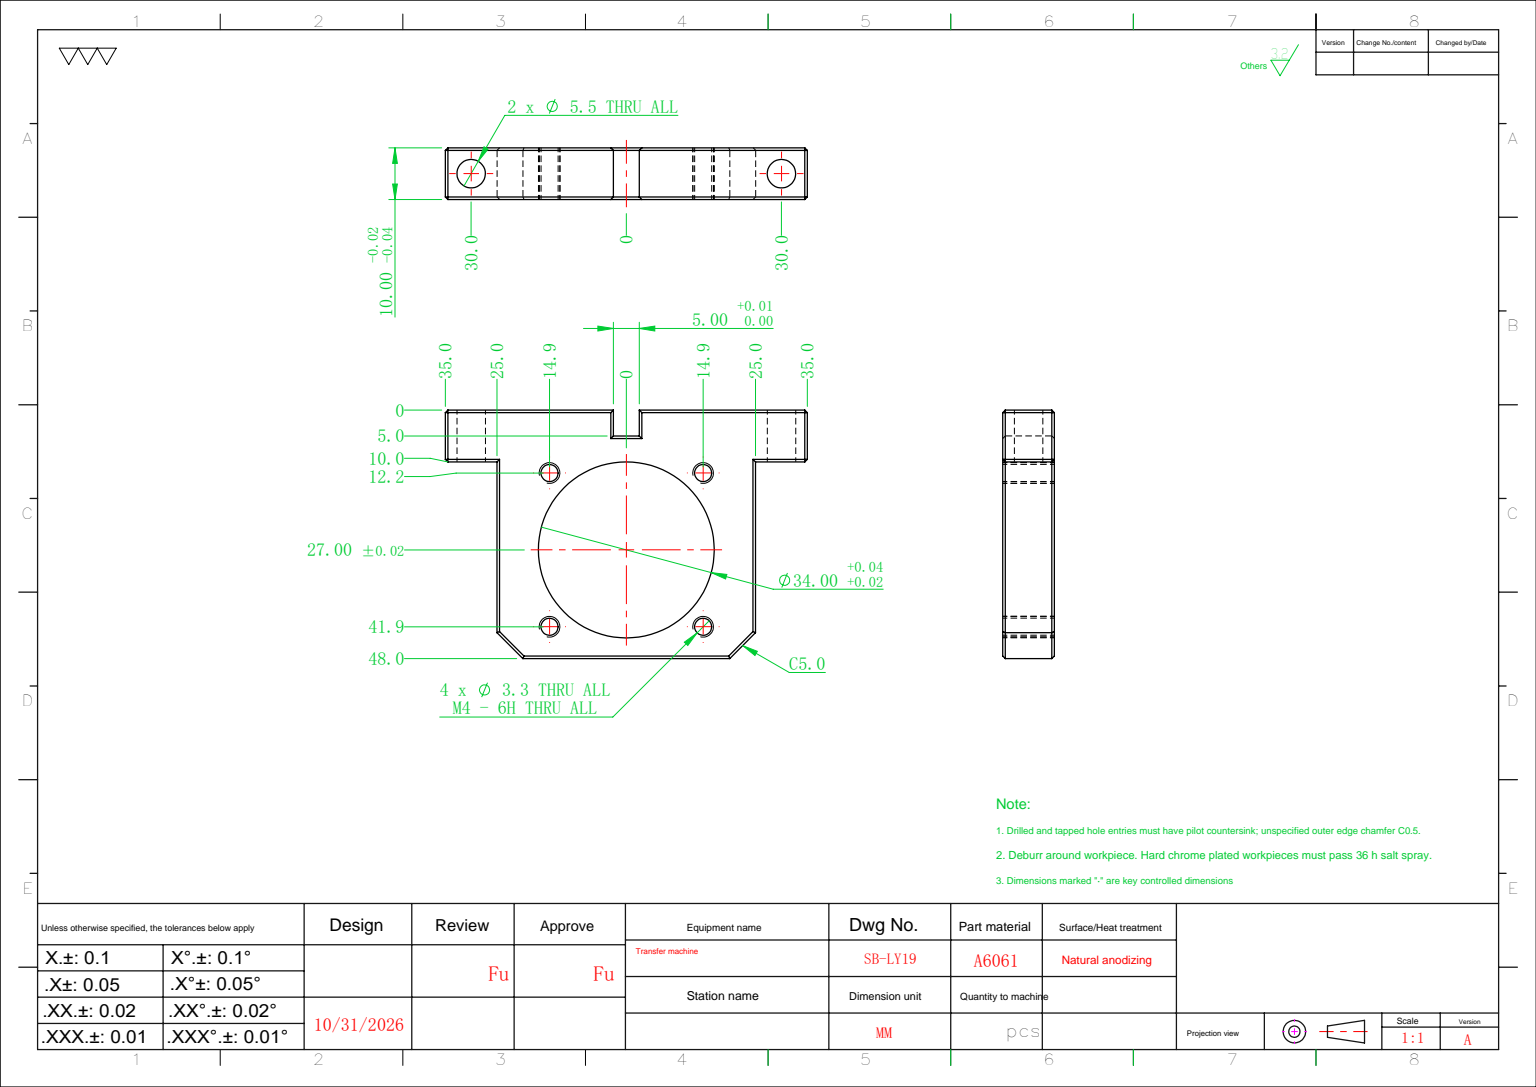
from build123d import *

# Parameters (mm, degrees)
SKETCH_1_W              = 70
SKETCH_1_H              = 48
EXTRUDE_1_DEPTH         = 10
SKETCH_2_W              = 10
SKETCH_2_H              = 38
CUT_EXTRUDE_1_DEPTH     = 44.600458713
SKETCH_3_R              = 17
CUT_EXTRUDE_2_DEPTH     = 44.600458713
HOLE_WIZARD_M4_2_D      = 3.3
HOLE_WIZARD_5_5_5_5_1_D = 5.5
CHAMFER_1_SIZE          = 5
SKETCH_12_W             = 5
SKETCH_12_H             = 5
CUT_EXTRUDE_3_DEPTH     = 44.600458713
CHAMFER_2_SIZE          = 0.5


with BuildPart() as part:
    # 草图1 → 凸台-拉伸1 (new body)
    with BuildSketch(Plane.XY):
        Rectangle(SKETCH_1_W, SKETCH_1_H)
    extrude(amount=EXTRUDE_1_DEPTH)

    # 草图2 → 切除-拉伸1 (cut, through all)
    with BuildSketch(Plane.XY.offset(10)):
        with Locations((-30, -5)):
            Rectangle(SKETCH_2_W, SKETCH_2_H)
        with Locations((30, -5)):
            Rectangle(SKETCH_2_W, SKETCH_2_H)
    extrude(amount=-CUT_EXTRUDE_1_DEPTH, mode=Mode.SUBTRACT)

    # 草图3 → 切除-拉伸2 (cut, through all)
    with BuildSketch(Plane(origin=(0, 0, 0), x_dir=(-1, 0, 0), z_dir=(0, 0, -1))):
        with Locations((0, -3)):
            Circle(SKETCH_3_R)
    extrude(amount=-CUT_EXTRUDE_2_DEPTH, mode=Mode.SUBTRACT)

    # M4 螺纹孔2 (through all)
    with Locations(Plane.XY.offset(10)):
        with Locations((14.85, -17.85), (-14.85, -17.85), (-14.85, 11.85), (14.85, 11.85)):
            Hole(HOLE_WIZARD_M4_2_D / 2)

    # Ø5.5 (5.5) 直径孔1 (through all)
    with Locations(Plane(origin=(0, 14, 0), x_dir=(-1, 0, 0), z_dir=(0, -1, 0))):
        with Locations((-30, -5), (30, -5)):
            Hole(HOLE_WIZARD_5_5_5_5_1_D / 2)

    # 倒角1
    chamfer_1_edges = [part.edges().sort_by_distance(p)[0] for p in [
        (-25, -24, 5),
        (25, -24, 5),
    ]]
    chamfer(chamfer_1_edges, length=CHAMFER_1_SIZE)

    # 草图12 → 切除-拉伸3 (cut, through all)
    with BuildSketch(Plane.XY.offset(10)):
        with Locations((0, 21.5)):
            Rectangle(SKETCH_12_W, SKETCH_12_H)
    extrude(amount=-CUT_EXTRUDE_3_DEPTH, mode=Mode.SUBTRACT)

    # 倒角2
    chamfer_2_edges = [part.edges().sort_by_distance(p)[0] for p in [
        (-35, 19, 10),
        (-30, 14, 0),
        (-35, 14, 5),
        (-30, 14, 10),
        (35, 19, 0),
        (35, 19, 10),
        (25, -2.5, 0),
        (30, 14, 0),
        (35, 14, 5),
        (30, 14, 10),
        (25, -2.5, 10),
        (-35, 19, 0),
        (18.75, 24, 0),
        (18.75, 24, 10),
        (-35, 24, 5),
        (35, 24, 5),
        (-25, -2.5, 10),
        (-25, -2.5, 0),
        (0, -24, 10),
        (22.5, -21.5, 10),
        (-22.5, -21.5, 10),
        (0, -24, 0),
        (22.5, -21.5, 0),
        (-22.5, -21.5, 0),
        (-18.75, 24, 0),
        (-18.75, 24, 10),
        (-2.5, 21.5, 0),
        (2.5, 21.5, 0),
        (0, 19, 0),
        (-2.5, 21.5, 10),
        (0, 19, 10),
        (2.5, 21.5, 10),
    ]]
    chamfer(chamfer_2_edges, length=CHAMFER_2_SIZE)


solid = part.part
